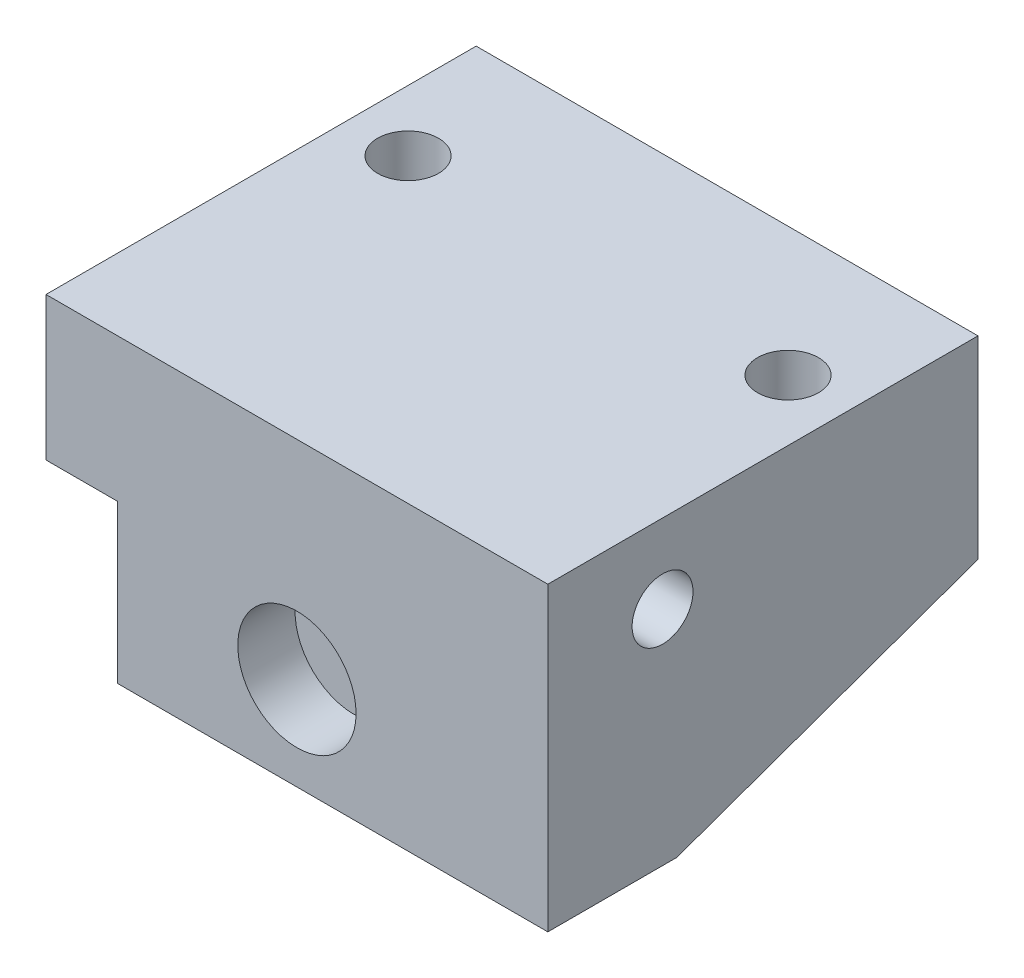
from build123d import *

# Parameters (mm, degrees)
SKETCH1_W           = 70
SKETCH1_H           = 60
BOSS_EXTRUDE1_DEPTH = 20
BOSS_EXTRUDE2_DEPTH = 60
SKETCH5_R           = 4.25
CUT_EXTRUDE3_DEPTH  = 131
SKETCH7_R           = 4.25
CUT_EXTRUDE4_DEPTH  = 91
SKETCH8_R           = 8.25
CUT_EXTRUDE5_DEPTH  = 8


with BuildPart() as part:
    # Sketch1 → Boss-Extrude1 (new body)
    with BuildSketch(Plane(origin=(0, 0, 0), x_dir=(1, 0, 0), z_dir=(0, 1, 0))):
        Rectangle(SKETCH1_W, SKETCH1_H)
    extrude(amount=BOSS_EXTRUDE1_DEPTH)

    # Sketch2 → Boss-Extrude2 (add)
    with BuildSketch(Plane(origin=(35, 0, 0), x_dir=(0, 0, -1), z_dir=(1, 0, 0))):
        Polygon((30, 20), (30, 0), (30, -7), (-12, -22), (-30, -22), (-30, 20), align=None)
    extrude(amount=-BOSS_EXTRUDE2_DEPTH)

    # Sketch5 → Cut-Extrude3 (cut)
    with BuildSketch(Plane.ZY.offset(35)):
        with Locations((14, 9)):
            Circle(SKETCH5_R)
    extrude(amount=-CUT_EXTRUDE3_DEPTH, mode=Mode.SUBTRACT)

    # Sketch7 → Cut-Extrude4 (cut)
    with BuildSketch(Plane(origin=(0, 20, 0), x_dir=(1, 0, 0), z_dir=(0, 1, 0))):
        with Locations(Location((26.5, 12, 0), (0, 0, 270))):
            Circle(SKETCH7_R)
        with Locations(Location((-26.5, 12, 0), (0, 0, 290.667316494))):
            Circle(SKETCH7_R)
    extrude(amount=-CUT_EXTRUDE4_DEPTH, mode=Mode.SUBTRACT)

    # Sketch8 → Cut-Extrude5 (cut)
    with BuildSketch(Plane.XY.offset(30)):
        with Locations((0, -9)):
            Circle(SKETCH8_R)
    extrude(amount=-CUT_EXTRUDE5_DEPTH, mode=Mode.SUBTRACT)


solid = part.part
